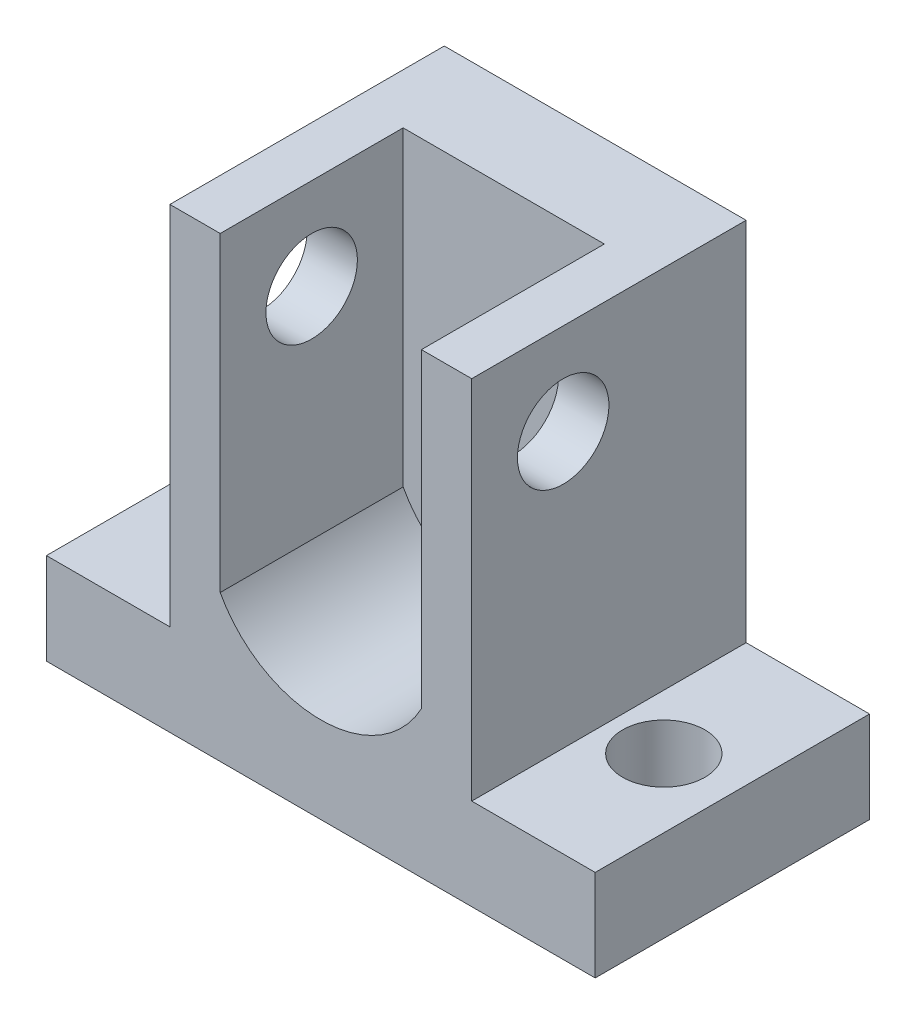
SolidWorks part; units mm, degrees
ref_plane "Front Plane" through (0, 0, 0) normal (0, 0, 1) x (1, 0, 0)
ref_plane "Top Plane" through (0, 0, 0) normal (0, 1, 0) x (1, 0, 0)
ref_plane "Right Plane" through (0, 0, 0) normal (1, 0, 0) x (0, 0, -1)
ref_plane "Plane4" through (0, 0, 30) normal (0, 0, 1) x (1, 0, 0)
sketch "Sketch1" plane through (0, 0, 30) normal (0, 0, 1) x (1, 0, 0)
  line L0 (60, 50) -> (0, 50)
  line L1 (0, 50) -> (0, 0)
  line L2 (0, 0) -> (60, 0)
  line L3 (60, 0) -> (60, 50)
  dimension "D1" = 50
  dimension "D2" = 60
extrude "Boss-Extrude1" add sketch "Sketch1" against normal blind 30
sketch "Sketch2" plane through (0, 0, 0) normal (0, 0, -1) x (-1, 0, 0)
  line L0 (-60, 10) -> (-46.5, 10)
  line L1 (-46.5, 10) -> (-46.5, 50)
  line L2 (-46.5, 50) -> (-60, 50)
  line L3 (-60, 50) -> (-60, 10)
  line L6 (-60, 0) -> (-60, 50) construction
  dimension "D1" = 13.5
  dimension "D2" = 40
extrude "Cut-Extrude1" cut sketch "Sketch2" against normal through all
sketch "Sketch3" plane through (0, 0, 0) normal (0, 0, -1) x (-1, 0, 0)
  line L0 (-13.5, 50) -> (-13.5, 10)
  line L1 (-13.5, 10) -> (0, 10)
  line L2 (0, 10) -> (0, 50)
  line L3 (0, 50) -> (-13.5, 50)
  line L4 (0, 50) -> (0, 0) construction
  dimension "D1" = 13.5
extrude "Cut-Extrude2" cut sketch "Sketch3" against normal through all
sketch "Sketch4" plane through (0, 0, 30) normal (0, 0, 1) x (1, 0, 0)
  line L0 (19, 50) -> (19, 16)
  line L1 (41, 16) -> (41, 50)
  line L2 (41, 50) -> (19, 50)
  line L3 (46.5, 50) -> (13.5, 50) construction
  line L4 (30, 0) -> (30, 50) construction
  line L5 (0, 0) -> (60, 0) construction
  arc A1 (19, 16) -> (41, 16) centre (30, 21.9372) ccw
  dimension "D2" = 34
  dimension "D3" = 12.5
  dimension "D1" = 22
extrude "Cut-Extrude3" cut sketch "Sketch4" against normal blind 20
hole_wizard "Ø9.0 (9) Diameter Hole1" positions "Sketch6" profile "Sketch5" hole size "Ø9.0" standard "ANSI Metric" end condition through all
sketch "Sketch6" plane through (0, 0, 0) normal (0, -1, 0) x (-1, 0, 0)
  line L0 (0, 0) -> (0, -30) construction
  line L1 (-60, 0) -> (-60, -30) construction
  point P0 (-7.5, -15)
  point P1 (-52.5, -15)
  dimension "D1" = 7.5
  dimension "D2" = 7.5
sketch "Sketch5" plane through (7.5, 0, 15) normal (1, 0, 0) x (0, 0, -1)
  line L0 (0, 0) -> (0, 50)
  line L1 (0, 50) -> (4.5, 50)
  line L2 (4.5, 50) -> (4.5, 0)
  line L5 (4.5, 0) -> (0, 0)
  line L11 (0, -6.35) -> (0, 107.95) construction
  dimension "通孔孔直径" = 9
  dimension "通孔孔深度" = 50
hole_wizard "Ø10.0 (10) Diameter Hole1" positions "Sketch8" profile "Sketch7" hole size "Ø10.0" standard "ANSI Metric"
sketch "Sketch8" plane through (41, 0, 0) normal (-1, 0, 0) x (0, 0, 1)
  point P0 (20, 40)
sketch "Sketch7" plane through (41, 40, 20) normal (0, 1, 0) x (0, 0, 1)
  line L0 (0, 0) -> (0, 19)
  line L1 (0, 19) -> (5, 19)
  line L2 (5, 19) -> (5, 0)
  line L5 (5, 0) -> (0, 0)
  line L11 (0, -6.35) -> (0, 107.95) construction
  dimension "通孔孔直径" = 10
  dimension "通孔孔深度" = 19
hole_wizard "Ø10.0 (10) Diameter Hole2" positions "Sketch10" profile "Sketch9" hole size "Ø10.0" standard "ANSI Metric"
sketch "Sketch10" plane through (19, 0, 0) normal (1, 0, 0) x (0, 0, -1)
  point P0 (-20, 40)
sketch "Sketch9" plane through (19, 40, 20) normal (0, 1, 0) x (0, 0, -1)
  line L0 (0, 0) -> (0, 19)
  line L1 (0, 19) -> (5, 19)
  line L2 (5, 19) -> (5, 0)
  line L5 (5, 0) -> (0, 0)
  line L11 (0, -6.35) -> (0, 107.95) construction
  dimension "通孔孔直径" = 10
  dimension "通孔孔深度" = 19
